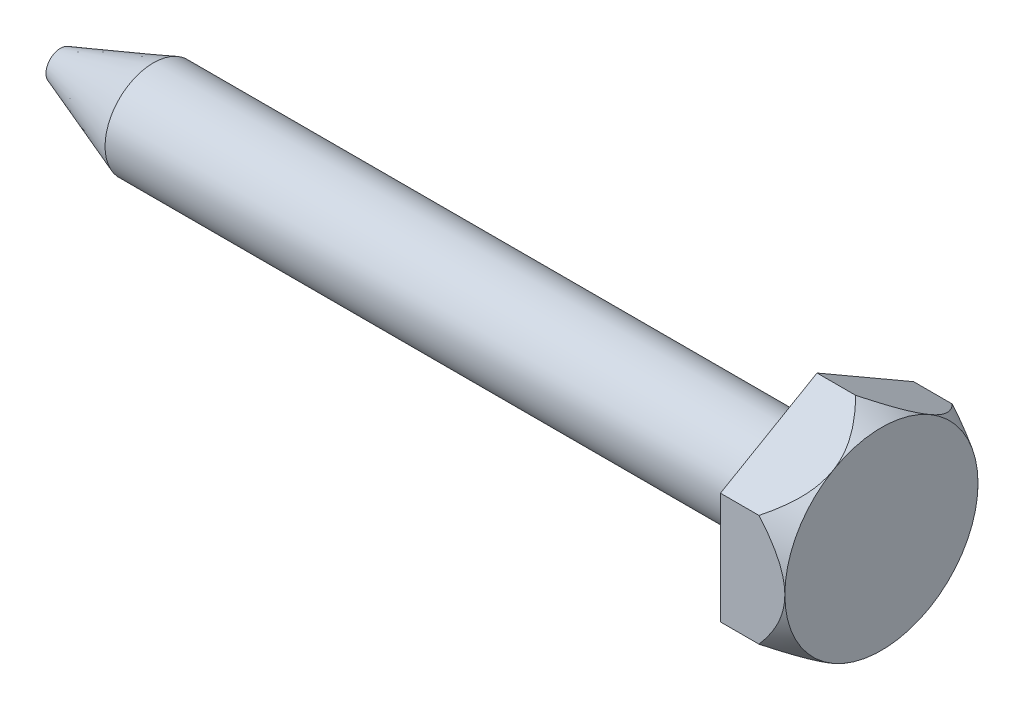
from build123d import *

# Parameters (mm, degrees)
BOSS_EXTRUDE1_DEPTH = 4
SKETCH2_OUTSIDE_W   = 40.846
SKETCH2_OUTSIDE_H   = 42.702
SKETCH2_OUTSIDE_R   = 6
CUT_EXTRUDE1_DEPTH  = 20
CUT_EXTRUDE1_DRAFT  = -30


with BuildPart() as part:
    # Sketch1 → Boss-Extrude1 (new body)
    with BuildSketch(Plane(origin=(0, 0, 0), x_dir=(0, 0, -1), z_dir=(1, 0, 0))):
        Polygon((0, -6.92820323), (6, -3.464101615), (6, 3.464101615), (0, 6.92820323), (-6, 3.464101615), (-6, -3.464101615), align=None)
    extrude(amount=BOSS_EXTRUDE1_DEPTH)


with BuildPart() as cut_extrude1_tool:
    # Sketch2 outside → Cut-Extrude1 (with draft: the straight prism first)
    with BuildSketch(Plane(origin=(4, 0, 0), x_dir=(0, 0, -1), z_dir=(1, 0, 0))):
        Rectangle(SKETCH2_OUTSIDE_W, SKETCH2_OUTSIDE_H)
        Circle(SKETCH2_OUTSIDE_R, mode=Mode.SUBTRACT)
    extrude(amount=-CUT_EXTRUDE1_DEPTH)
    # Cut-Extrude1: the draft: its side faces are tilted about the plane it starts from
    cut_extrude1_sides = [cut_extrude1_tool.faces().sort_by_distance(p)[0] for p in [
        (-6, -21.351, 0),
        (-6, 0, -20.423),
        (-6, 21.351, 0),
        (-6, 0, 20.423),
        (-6, 0, 6),
    ]]
    draft(cut_extrude1_sides, Plane(origin=(4, 0, 0), x_dir=(0, 0, -1), z_dir=(1, 0, 0)), CUT_EXTRUDE1_DRAFT)


with BuildPart() as part_1:
    add(part.part)

    # Cut-Extrude1: cut by cut_extrude1_tool
    add(cut_extrude1_tool.part, mode=Mode.SUBTRACT)

    # Sketch3 → Revolve1 (revolve)
    with BuildSketch(Plane.XY, mode=Mode.PRIVATE) as revolve1_sk:
        Polygon((0, 0), (0, 3), (-41.230297419, 3), (-47, 0.9), (-47, 0), align=None)
    revolve(revolve1_sk.sketch.rotate(Axis((-32.199358367, 0, 0), (1, 0, 0)), 90), axis=Axis((-32.199358367, 0, 0), (1, 0, 0)))


solid = part_1.part
